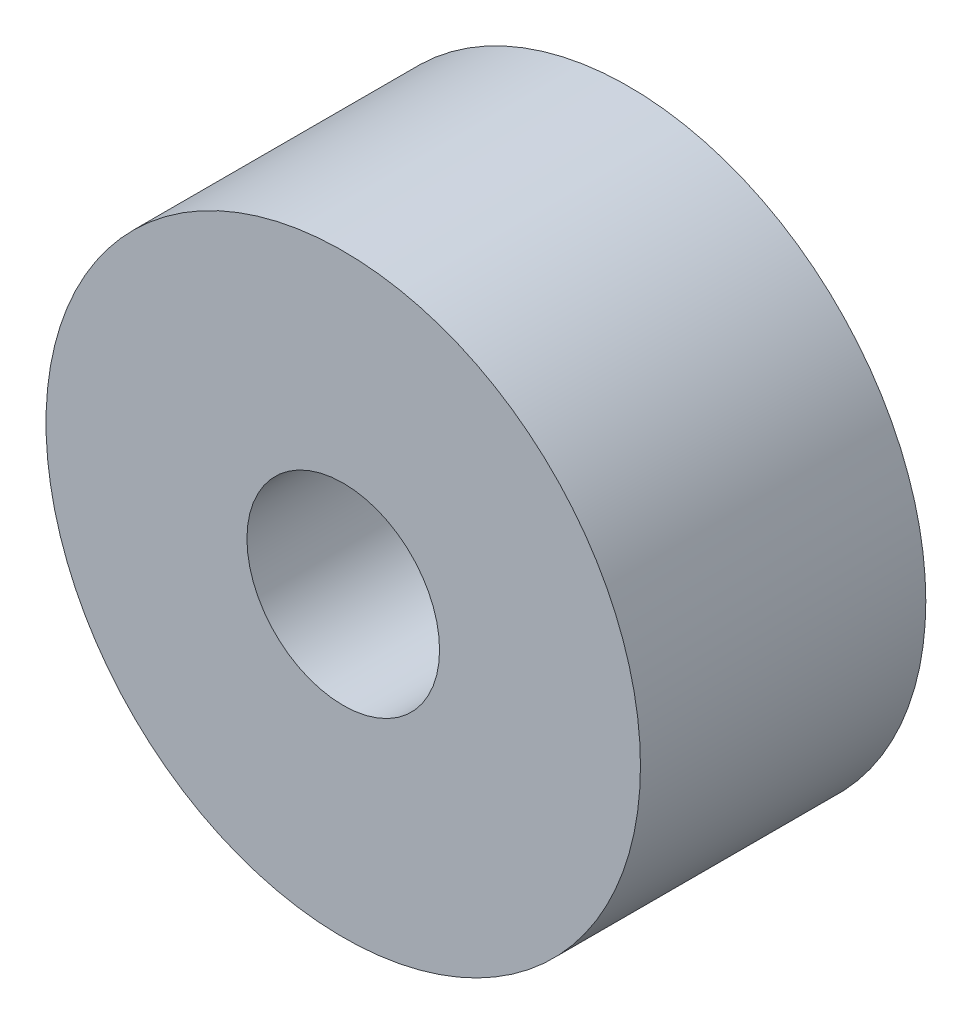
SolidWorks part; units mm, degrees
ref_plane "前视基准面" through (0, 0, 0) normal (0, 0, 1) x (1, 0, 0)
ref_plane "上视基准面" through (0, 0, 0) normal (0, 1, 0) x (1, 0, 0)
ref_plane "右视基准面" through (0, 0, 0) normal (1, 0, 0) x (0, 0, -1)
other "Configuration Table"
sketch "草图1" plane through (0, 0, 0) normal (0, 0, 1) x (1, 0, 0)
  circle A0 centre (0, 0) radius 25
  circle A1 centre (0, 0) radius 8.1
  point P0 (0, 0)
  dimension "D1" = 16.2
  dimension "D2" = 50
extrude "凸台-拉伸1" add sketch "草图1" against normal mid plane 24
